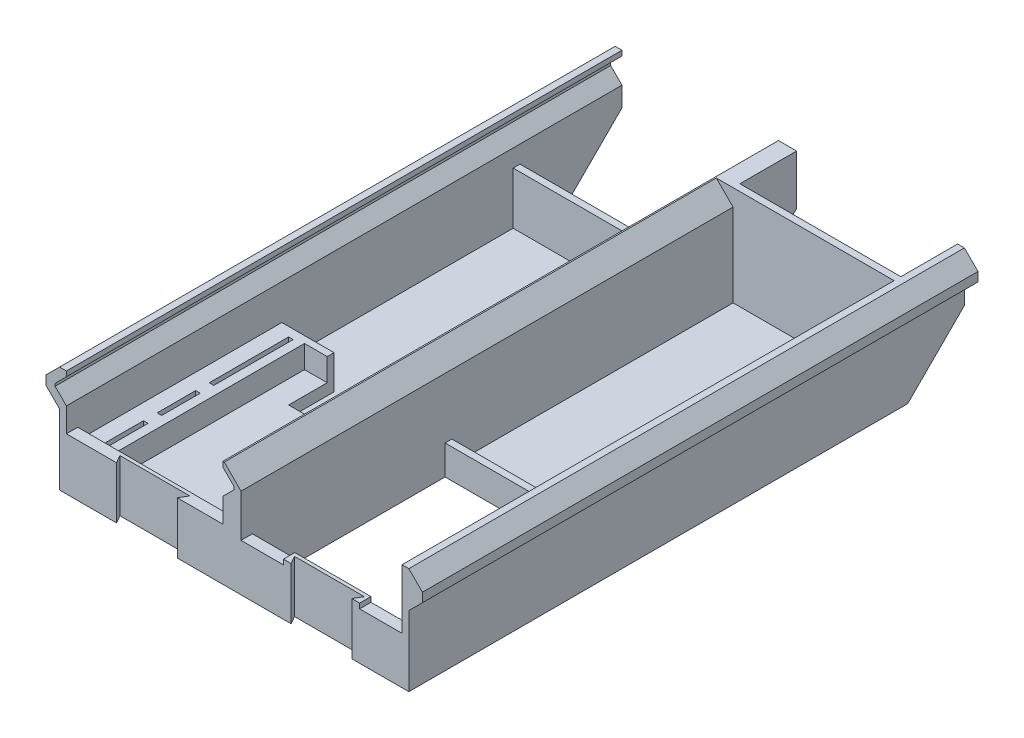
from build123d import *

# Parameters (mm, degrees)
BOSS_EXTRUDE1_DEPTH     = 200
SKETCH2_W               = 148
SKETCH2_H               = 194
CUT_EXTRUDE1_DEPTH      = 44
SKETCH4_W               = 8
SKETCH4_H               = 194
EXTRUDE_THIN1_DEPTH     = 44
CUT_EXTRUDE2_DEPTH      = 222.580685079
CUT_EXTRUDE3_DEPTH      = 219.876677606
MOVE_FACE1_BY           = 2
MOVE_FACE1_2_BY         = 2
CUT_EXTRUDE4_DEPTH      = 222.580685079
CUT_EXTRUDE5_DEPTH      = 16.595837
MOVE_FACE2_BY           = 45
MOVE_FACE3_BY           = 20
SKETCH9_W               = 71
SKETCH9_H               = 47
CUT_EXTRUDE6_DEPTH      = 25
SKETCH10_W              = 69
SKETCH10_H              = 26
CUT_EXTRUDE7_DEPTH      = 45
CUT_EXTRUDE8_DEPTH      = 45
CHAMFER1_SIZE           = 25
CUT_EXTRUDE9_REACH      = 264.393
SKETCH12_W              = 71
SKETCH12_H              = 85
SKETCH13_W              = 71
SKETCH13_H              = 3
BOSS_EXTRUDE2_DEPTH     = 10
SKETCH14_W              = 18.7
SKETCH14_H              = 5
CUT_EXTRUDE10_DEPTH     = 2.2
SKETCH15_W              = 69
SKETCH15_H              = 90
BOSS_EXTRUDE3_DEPTH     = 15
SKETCH16_W              = 56
SKETCH16_H              = 87
CUT_EXTRUDE11_DEPTH     = 10
CUT_EXTRUDE12_REACH     = 262.298
SKETCH17_W              = 36
SKETCH17_H              = 34
SKETCH18_W              = 2
SKETCH18_H              = 17
SKETCH18_H_2            = 35
CUT_EXTRUDE_THIN1_DEPTH = 7
MOVE_FACE4_BY           = 3


with BuildPart() as part:
    # Sketch1 → Boss-Extrude1 (new body)
    with BuildSketch(Plane.XY):
        Polygon((77, 0), (-77, 0), (-77, 31), (-83, 37), (-83, 41), (-77, 47), (77, 47), (83, 41), (83, 37), (77, 31), align=None)
    extrude(amount=-BOSS_EXTRUDE1_DEPTH)

    # Sketch2 → Cut-Extrude1 (cut)
    with BuildSketch(Plane(origin=(0, 47, 0), x_dir=(1, 0, 0), z_dir=(0, 1, 0))):
        with Locations((0, 100)):
            Rectangle(SKETCH2_W, SKETCH2_H)
    extrude(amount=-CUT_EXTRUDE1_DEPTH, mode=Mode.SUBTRACT)

    # Sketch4 → Extrude-Thin1 (add)
    with BuildSketch(Plane(origin=(0, 3, 0), x_dir=(1, 0, 0), z_dir=(0, 1, 0))):
        with Locations((-1, 100)):
            Rectangle(SKETCH4_W, SKETCH4_H)
    extrude(amount=EXTRUDE_THIN1_DEPTH)

    # Sketch5 → Cut-Extrude2 (cut, through all)
    with BuildSketch(Plane.XY):
        Polygon((-74, 47), (-74, 44.767409819), (-79, 39.767409819), (-79, 38.656854249), (-74, 33.656854249), (-74, 26), (-5, 26), (-5, 33.656854249), (0, 38.656854249), (0, 39.767409819), (-5, 44.767409819), (-5, 47), align=None)
    extrude(amount=-CUT_EXTRUDE2_DEPTH, mode=Mode.SUBTRACT)

    # Sketch6 → Cut-Extrude3 (cut, through all)
    with BuildSketch(Plane.XY.offset(-197)):
        Polygon((-4.404163056, 47), (3, 39.595836944), (74, 39.595836944), (74, 47), (3, 47), align=None)
    extrude(amount=CUT_EXTRUDE3_DEPTH, mode=Mode.SUBTRACT)

    # Move Face1: a face moved outward by 2.0
    extrude(part.faces().sort_by_distance((-39.5, 14.5, -3))[0], amount=MOVE_FACE1_BY, dir=(0, 0, -1))

    # Move Face1 2: a face moved outward by 2.0
    extrude(part.faces().sort_by_distance((38.5, 21.297918472, -3))[0], amount=MOVE_FACE1_2_BY, dir=(0, 0, -1))

    # Sketch7 → Cut-Extrude4 (cut, through all)
    with BuildSketch(Plane.XZ):
        Polygon((-51.883419246, 0), (-53.904145188, -3.5), (-23.095854812, -3.5), (-25.116580754, 0), align=None)
        Polygon((25.116580754, 0), (51.883419246, 0), (53.904145188, -3.5), (23.095854812, -3.5), align=None)
    extrude(amount=-CUT_EXTRUDE4_DEPTH, mode=Mode.SUBTRACT)

    # Sketch8 → Cut-Extrude5 (cut)
    with BuildSketch(Plane(origin=(0, 39.595836944, 0), x_dir=(1, 0, 0), z_dir=(0, 1, 0))):
        Polygon((25.116580754, 0), (23.095854812, 3.5), (53.904145188, 3.5), (51.883419246, 0), (74, 0), (74, 5), (3, 5), (3, 0), align=None)
        Polygon((-53.904145188, 3.5), (-23.095854812, 3.5), (-25.116580754, 0), (-5, 0), (-5, 5), (-74, 5), (-74, 0), (-51.883419246, 0), align=None)
    extrude(amount=-CUT_EXTRUDE5_DEPTH, mode=Mode.SUBTRACT)

    # Move Face2: a face moved outward by 45.0
    extrude(part.faces().sort_by_distance((10.200110487, 20.43272532, -200))[0], amount=MOVE_FACE2_BY, dir=(0, 0, -1))

    # Move Face3: a face moved inward by 20.0
    extrude(part.faces().sort_by_distance((38.169755743, 25.169887896, -197))[0], amount=MOVE_FACE3_BY, dir=(0, 0, -1), mode=Mode.SUBTRACT)

    # Sketch9 → Cut-Extrude6 (cut)
    with BuildSketch(Plane(origin=(0, 0, -245), x_dir=(-1, 0, 0), z_dir=(0, 0, -1))):
        with Locations((-38.5, 23.5)):
            Rectangle(SKETCH9_W, SKETCH9_H)
    extrude(amount=-CUT_EXTRUDE6_DEPTH, mode=Mode.SUBTRACT)

    # Sketch10 → Cut-Extrude7 (cut)
    with BuildSketch(Plane(origin=(0, 0, -245), x_dir=(-1, 0, 0), z_dir=(0, 0, -1))):
        with Locations((39.5, 13)):
            Rectangle(SKETCH10_W, SKETCH10_H)
    extrude(amount=-CUT_EXTRUDE7_DEPTH, mode=Mode.SUBTRACT)

    # Sketch11 → Cut-Extrude8 (cut)
    with BuildSketch(Plane(origin=(0, 0, -245), x_dir=(-1, 0, 0), z_dir=(0, 0, -1))):
        Polygon((5, 0), (5, 30.656854249), (0, 25.656854249), (0, 0), align=None)
    extrude(amount=-CUT_EXTRUDE8_DEPTH, mode=Mode.SUBTRACT)

    # Chamfer1
    chamfer1_edges = [part.edges().sort_by_distance(p)[0] for p in [
        (-75.5, 0, -245),
        (1.5, 0, -245),
        (75.5, 0, -245),
    ]]
    chamfer(chamfer1_edges, length=CHAMFER1_SIZE)

    # Sketch12 → Cut-Extrude9 (cut, up to next)
    with BuildSketch(Plane(origin=(0, 3, 0), x_dir=(1, 0, 0), z_dir=(0, 1, 0)), mode=Mode.PRIVATE) as cut_extrude9_sk1:
        with Locations((38.5, 47.5)):
            Rectangle(SKETCH12_W, SKETCH12_H)
    cut_extrude9_tool1 = extrude(cut_extrude9_sk1.sketch, amount=-CUT_EXTRUDE9_REACH, mode=Mode.PRIVATE) & part.part
    add(cut_extrude9_tool1.solids().sort_by_distance((38.5, 3, -47.5))[0], mode=Mode.SUBTRACT)

    # Sketch13 → Boss-Extrude2 (add)
    with BuildSketch(Plane(origin=(0, 3, 0), x_dir=(1, 0, 0), z_dir=(0, 1, 0))):
        with Locations((38.5, 91.5)):
            Rectangle(SKETCH13_W, SKETCH13_H)
    extrude(amount=BOSS_EXTRUDE2_DEPTH)

    # Sketch14 → Cut-Extrude10 (cut)
    with BuildSketch(Plane(origin=(0, 23, 0), x_dir=(1, 0, 0), z_dir=(0, 1, 0))):
        with Locations((12.35, 2.5)):
            Rectangle(SKETCH14_W, SKETCH14_H)
        with Locations((64.65, 2.5)):
            Rectangle(SKETCH14_W, SKETCH14_H)
    extrude(amount=-CUT_EXTRUDE10_DEPTH, mode=Mode.SUBTRACT)

    # Sketch15 → Boss-Extrude3 (add)
    with BuildSketch(Plane(origin=(0, 3, 0), x_dir=(1, 0, 0), z_dir=(0, 1, 0))):
        with Locations((-39.5, 50)):
            Rectangle(SKETCH15_W, SKETCH15_H)
    extrude(amount=BOSS_EXTRUDE3_DEPTH)

    # Sketch16 → Cut-Extrude11 (cut)
    with BuildSketch(Plane(origin=(0, 18, 0), x_dir=(1, 0, 0), z_dir=(0, 1, 0))):
        with Locations((-33, 48.5)):
            Rectangle(SKETCH16_W, SKETCH16_H)
    extrude(amount=-CUT_EXTRUDE11_DEPTH, mode=Mode.SUBTRACT)

    # Cut-Extrude12: up to this face of the body (flat: up to its plane)
    cut_extrude12_end = Plane(part.part.faces().sort_by_distance((-39.5, 3, -146))[0])
    # Sketch17 → Cut-Extrude12 (cut, up to the picked face)
    with BuildSketch(Plane(origin=(0, 18, 0), x_dir=(1, 0, 0), z_dir=(0, 1, 0)), mode=Mode.PRIVATE) as cut_extrude12_sk1:
        with Locations((-33, 92)):
            Rectangle(SKETCH17_W, SKETCH17_H)
    cut_extrude12_tool1 = split(extrude(cut_extrude12_sk1.sketch, amount=-CUT_EXTRUDE12_REACH, mode=Mode.PRIVATE), bisect_by=cut_extrude12_end, keep=Keep.BOTH, mode=Mode.PRIVATE)
    add(cut_extrude12_tool1.solids().sort_by(Axis((-33, 18, -92), (0, -1, 0)))[0], mode=Mode.SUBTRACT)

    # Sketch18 → Cut-Extrude-Thin1 (cut)
    with BuildSketch(Plane(origin=(0, 18, 0), x_dir=(1, 0, 0), z_dir=(0, 1, 0))):
        with Locations((-66, 18.5)):
            Rectangle(SKETCH18_W, SKETCH18_H)
        with Locations((-66, 41.5)):
            Rectangle(SKETCH18_W, SKETCH18_H)
        with Locations((-66, 73.5)):
            Rectangle(SKETCH18_W, SKETCH18_H_2)
    extrude(amount=-CUT_EXTRUDE_THIN1_DEPTH, mode=Mode.SUBTRACT)

    # Move Face4: a face moved outward by 3.0
    extrude(part.faces().sort_by_distance((-66, 11, -73.5))[0], amount=MOVE_FACE4_BY, dir=(0, 1, 0))


solid = part.part
